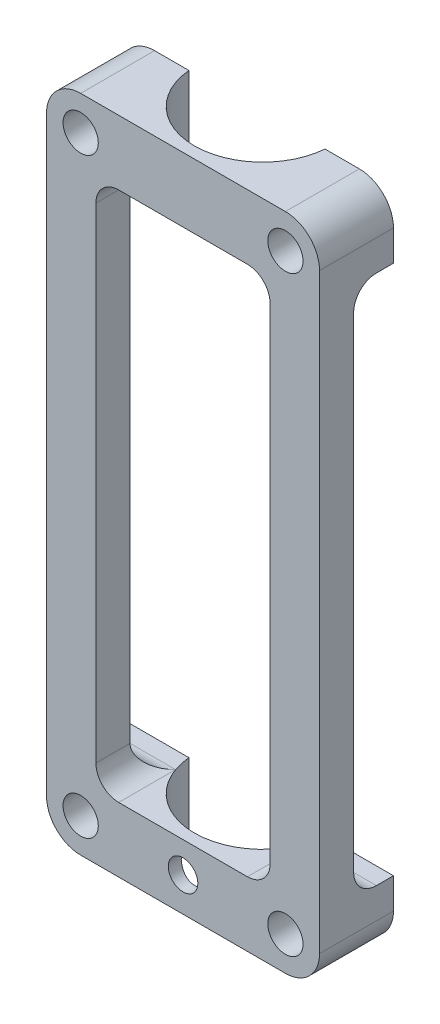
from build123d import *

# Parameters (mm, degrees)
EXTRUDE_1_DEPTH      = 7
EXTRUDE_1_DEPTH_BACK = 7
SKETCH_2_R           = 1.55
SKETCH_2_R_2         = 1.3
SKETCH_2_W           = 15.316718428
SKETCH_2_H           = 46.633436854
CUT_EXTRUDE_1_DEPTH  = 60.640590205
SKETCH_4_W           = 3.5
SKETCH_4_H           = 46.633436854
CUT_EXTRUDE_2_DEPTH  = 45.654227139
FILLET_1_R           = 2


with BuildPart() as part:
    # 草图2 → 凸台-拉伸1 (new, two sides: drawn at the far end of the back side and taken through both)
    with BuildSketch(Plane.XY.offset(-EXTRUDE_1_DEPTH_BACK)):
        with BuildLine():
            Line((9, 37), (-9, 37))
            ThreePointArc((-9, 37), (-11.121320344, 36.121320344), (-12, 34))
            Line((-12, 34), (-12, -18))
            ThreePointArc((-12, -18), (-11.121320344, -20.121320344), (-9, -21))
            Line((-9, -21), (9, -21))
            ThreePointArc((9, -21), (11.121320344, -20.121320344), (12, -18))
            Line((12, -18), (12, 34))
            ThreePointArc((12, 34), (11.121320344, 36.121320344), (9, 37))
        make_face()
        with Locations((-9, -18)):
            Circle(SKETCH_2_R, mode=Mode.SUBTRACT)
        with Locations((0, -18)):
            Circle(SKETCH_2_R_2, mode=Mode.SUBTRACT)
        with Locations((9, -18)):
            Circle(SKETCH_2_R, mode=Mode.SUBTRACT)
        with Locations((0, 8)):
            Rectangle(SKETCH_2_W, SKETCH_2_H, mode=Mode.SUBTRACT)
        with Locations((9, 34)):
            Circle(SKETCH_2_R, mode=Mode.SUBTRACT)
        with Locations((-9, 34)):
            Circle(SKETCH_2_R, mode=Mode.SUBTRACT)
    extrude(amount=EXTRUDE_1_DEPTH + EXTRUDE_1_DEPTH_BACK)

    # 草图3 → 切除-拉伸1 (cut, through all)
    with BuildSketch(Plane.XZ.offset(21)):
        with BuildLine():
            Line((-12, 0.5), (-5.979130372, 0.5))
            ThreePointArc((-5.979130372, 0.5), (0, 6), (5.979130372, 0.5))
            Line((5.979130372, 0.5), (12, 0.5))
            Line((12, 0.5), (12, -7))
            Line((12, -7), (-12, -7))
            Line((-12, -7), (-12, 0.5))
        make_face()
    extrude(amount=-CUT_EXTRUDE_1_DEPTH, mode=Mode.SUBTRACT)

    # 草图4 → 切除-拉伸2 (cut, through all)
    with BuildSketch(Plane.ZY.offset(12)):
        with Locations((2.25, 8)):
            Rectangle(SKETCH_4_W, SKETCH_4_H)
    extrude(amount=-CUT_EXTRUDE_2_DEPTH, mode=Mode.SUBTRACT)

    # 圆角1
    fillet_1_edges = [part.edges().sort_by_distance(p)[0] for p in [
        (7.658359214, 31.316718427, 5.5),
        (-7.658359214, 31.316718427, 5.5),
        (7.658359214, -15.316718427, 5.5),
        (-7.658359214, -15.316718427, 5.5),
        (-9.829179607, 31.316718427, 4),
        (-9.829179607, -15.316718427, 4),
        (9.829179607, -15.316718427, 4),
        (9.829179607, 31.316718427, 4),
    ]]
    fillet(fillet_1_edges, radius=FILLET_1_R)


solid = part.part
